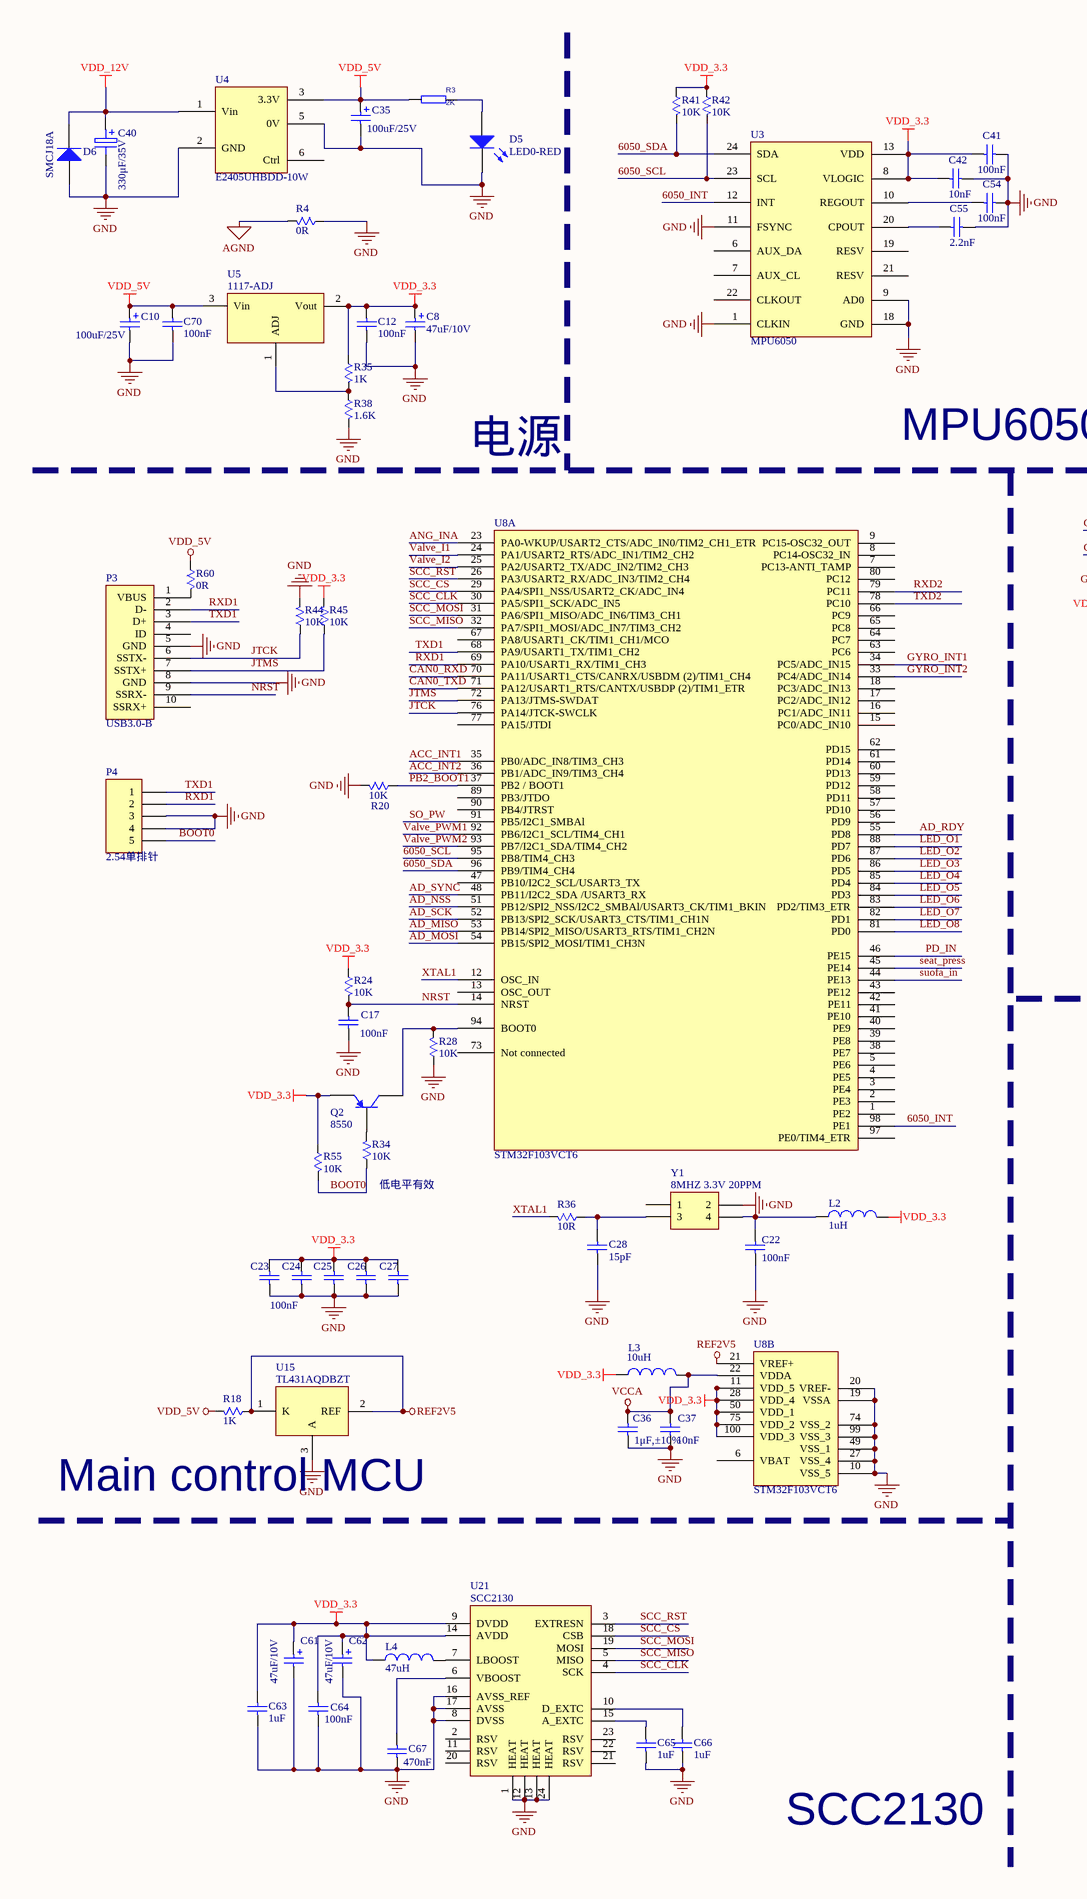
[diagram p0: MISC82155-6.SchDoc, left]
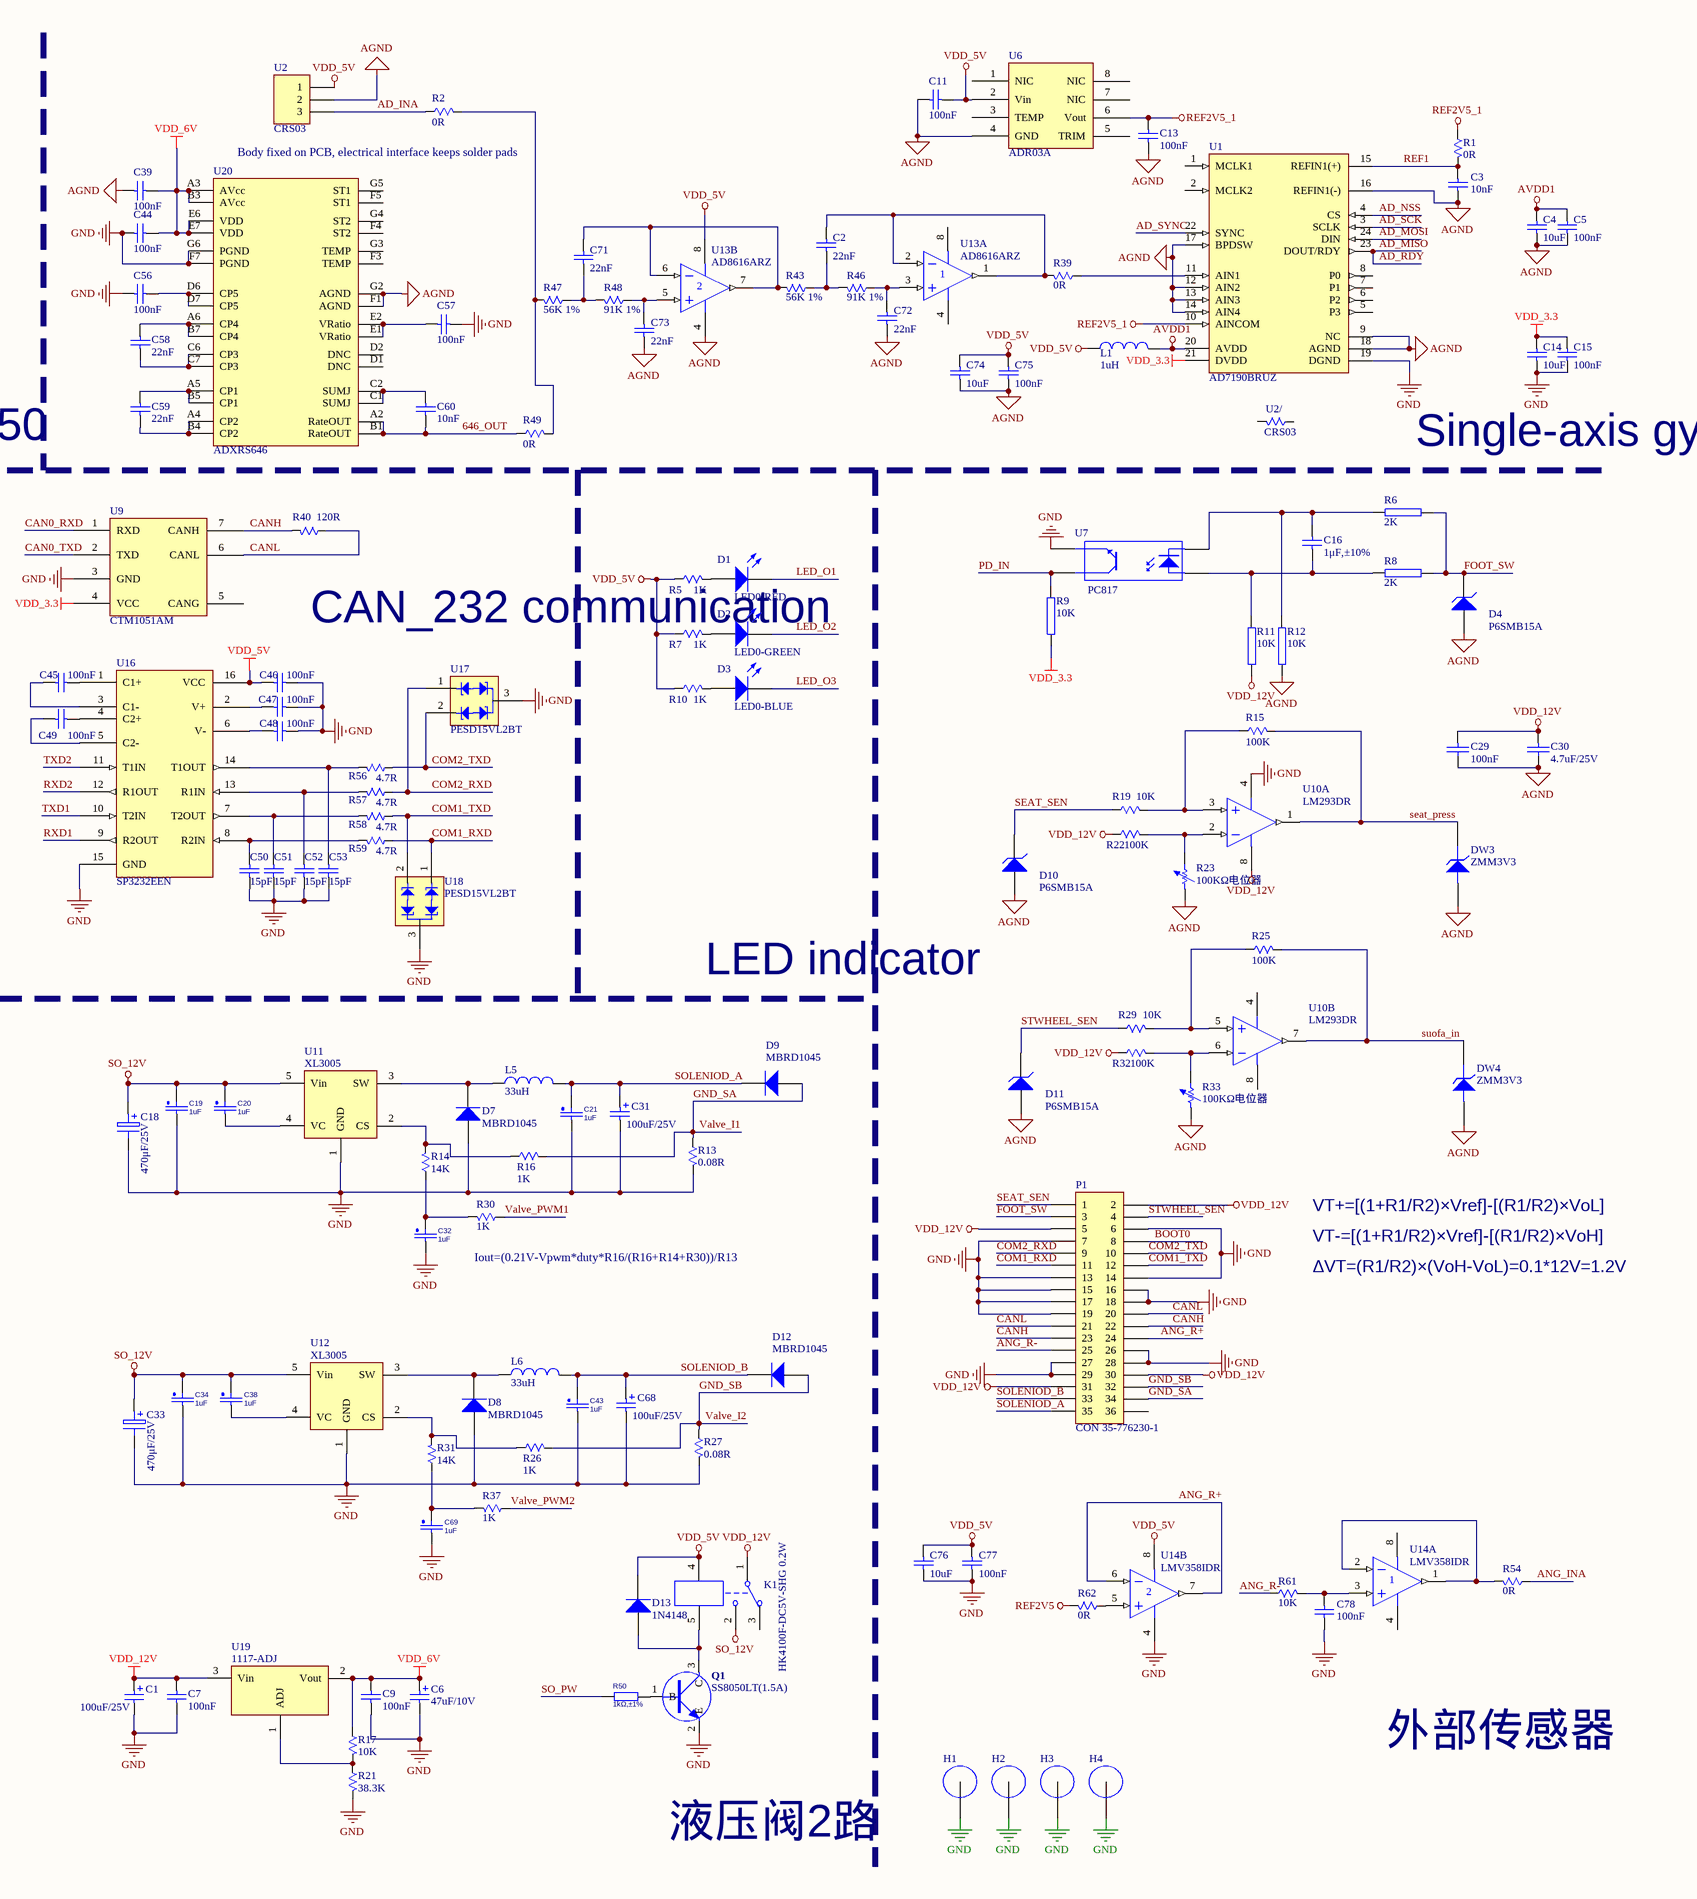
[diagram p1: MISC82155-6.SchDoc, right]
# Altium schematic sheet MISC82155-6.SchDoc
size A2

## Parts
C1  100uF/25V  [RB6.3*7]
C2  22nF  [C0805]
C3  10nF  [C0805]
C4  10uF  [C0805]
C5  100nF  [C0805]
C6  47uF/10V  [CT3528-B]
C7  100nF  [C0805]
C8  47uF/10V  [CT3528-B]
C9  100nF  [C0805]
C10  100uF/25V  [RB6.3*7]
C11  100nF  [C0805]
C12  100nF  [C0805]
C13  100nF  [C0805]
C14  10uF  [C0805]
C15  100nF  [C0805]
C16  1μF,±10%  [C0805]
C17  100nF  [C0805]
C18  470μF/25V  [CAPPR5.0-10X16-0.8]
C19  1uF  [C0805]
C20  1uF  [C0805]
C21  1uF  [C0805]
C22  100nF  [C0805]
C23  100nF  [C0805]
C24  100nF  [C0805]  (value not drawn)
C25  100nF  [C0805]  (value not drawn)
C26  100nF  [C0805]  (value not drawn)
C27  100nF  [C0805]  (value not drawn)
C28  15pF  [C0805]
C29  100nF  [C0805]
C30  4.7uF/25V  [1206C]
C31  100uF/25V  [RB6.3*7]
C32  1uF  [C0805]
C33  470μF/25V  [CAPPR5.0-10X16-0.8]
C34  1uF  [C0805]
C35  100uF/25V  [RB6.3*7]
C36  1μF,±10%  [C0805]
C37  10nF  [C0805]
C38  1uF  [C0805]
C39  100nF  [C0805]
C40  330μF/35V  [CAPPR5.0-10X16-0.8]
C41  100nF  [C0805]
C42  10nF  [C0805]
C43  1uF  [C0805]
C44  100nF  [C0805]
C45  100nF  [C0805]
C46  100nF  [C0805]
C47  100nF  [C0805]
C48  100nF  [C0805]
C49  100nF  [C0805]
C50  15pF  [C0805]
C51  15pF  [C0805]
C52  15pF  [C0805]
C53  15pF  [C0805]
C54  100nF  [C0805]
C55  2.2nF  [C0805]
C56  100nF  [C0805]
C57  100nF  [C0805]
C58  22nF  [C0805]
C59  22nF  [C0805]
C60  10nF  [C0805]
C61  47uF/10V  [CT3528-B]
C62  47uF/10V  [CT3528-B]
C63  1uF  [C0805]
C64  100nF  [C0805]
C65  1uF  [C0805]
C66  1uF  [C0805]
C67  470nF  [C0805]
C68  100uF/25V  [RB6.3*7]
C69  1uF  [C0805]
C70  100nF  [C0805]
C71  22nF  [C0805]
C72  22nF  [C0805]
C73  22nF  [C0805]
C74  10uF  [C0805]
C75  100nF  [C0805]
C76  10uF  [C0805]
C77  100nF  [C0805]
C78  100nF  [C0805]
D1  LED0-RED  [LED0805]
D2  LED0-GREEN  [LED0805]
D3  LED0-BLUE  [LED0805]
D4  P6SMB15A  [DO-214]
D5  LED0-RED  [LED0805]
D6  SMCJ18A  [SMC]
D7  MBRD1045  [TO-252]
D8  MBRD1045  [TO-252]
D9  MBRD1045  [TO-252]
D10  P6SMB15A  [DO-214]
D11  P6SMB15A  [DO-214]
D12  MBRD1045  [TO-252]
D13  1N4148  [SMD-D4148]
DW3  ZMM3V3  [SMD-D4148]
DW4  ZMM3V3  [SMD-D4148]
H1  Hole  [HOLE-3.2]  (value not drawn)
H2  Hole  [HOLE-3.2]  (value not drawn)
H3  Hole  [HOLE-3.2]  (value not drawn)
H4  Hole  [HOLE-3.2]  (value not drawn)
K1  HK4100F-DC5V-SHG 0.2W  [HK4100F]
L1  1uH  [R0805]
L2  1uH  [R0805]
L3  10uH  [R0805]
L4  47uH  [R1210]
L5  33uH  [SLF12555]
L6  33uH  [SLF12555]
P1  CON 35-776230-1  [VGA35]
P3  USB3.0-B  [Micro USB3.0-B]
P4  2.54单排针  [HDR1X5]
Q1  SS8050LT(1.5A)  [SOT-23]
Q2  8550  [SOT-23]
R1  0R  [R0805]
R2  0R  [R0805]
R3  2K  [R0805]
R4  0R  [R0805]
R5  1K  [R0805]
R6  2K  [R0805]
R7  1K  [R0805]
R8  2K  [R0805]
R9  10K  [R0805]
R10  1K  [R0805]
R11  10K  [R0805]
R12  10K  [R0805]
R13  0.08R  [R2512]
R14  14K  [R0805]
R15  100K  [R0805]
R16  1K  [R0805]
R17  10K  [R0805]
R18  1K  [R0805]
R19  10K  [R0805]
R20  10K  [R0805]
R21  38.3K  [R0805]
R22  100K  [R0805]
R23  100KΩ电位器  [CHANGER3]
R24  10K  [R0805]
R25  100K  [R0805]
R26  1K  [R0805]
R27  0.08R  [R2512]
R28  10K  [R0805]
R29  10K  [R0805]
R30  1K  [R0805]
R31  14K  [R0805]
R32  100K  [R0805]
R33  100KΩ电位器  [CHANGER3]
R34  10K  [R0805]
R35  1K  [R0805]
R36  10R  [R0805]
R37  1K  [R0805]
R38  1.6K  [R0805]
R39  0R  [R0805]
R40  120R  [R0805]
R41  10K  [R0805]
R42  10K  [R0805]
R43  56K 1%  [R0805]
R44  10K  [R0805]
R45  10K  [R0805]
R46  91K 1%  [R0805]
R47  56K 1%  [R0805]
R48  91K 1%  [R0805]
R49  0R  [R0805]
R50  1kΩ,±1%  [0805R]
R54  0R  [R0805]
R55  10K  [R0805]
R56  4.7R  [R0805]
R57  4.7R  [R0805]
R58  4.7R  [R0805]
R59  4.7R  [R0805]
R60  0R  [R0805]
R61  10K  [R0805]
R62  0R  [R0805]
U1  AD7190BRUZ  [IC-24P-TSSOP-6_4MM-G]
U2  CRS03  [HDR1X3]
U2/  CRS03  [CDS43-01]
U3  MPU6050  [QFN24]
U4  E2405UHBDD-10W  [E2403UHBDD]
U5  1117-ADJ  [SOT-223]
U6  ADR03A  [SOP-8]
U7  PC817  [SMD-4]
U8  STM32F103VCT6  [QFP-100]  (parts A,B of 2)
U9  CTM1051AM  [CTM1051AM]
U10  LM293DR  [SOP-8]  (parts A,B of 2)
U11  XL3005  [TO-263-5]
U12  XL3005  [TO-263-5]
U13  AD8616ARZ  [SOP-8]  (parts A,B of 2)
U14  LMV358IDR  [SOP-8]  (parts A,B of 2)
U15  TL431AQDBZT  [LC-SOT-23(SOT-23-3)]
U16  SP3232EEN  [SOP16-6.6]
U17  PESD15VL2BT  [SOT-23]
U18  PESD15VL2BT  [SOT-23]
U19  1117-ADJ  [SOT-223]
U20  ADXRS646
U21  SCC2130  [SCC2130D]
Y1  8MHZ 3.3V 20PPM  [XTAL7050]

## Nets
AGND: C3.2 C4.2 C5.2 C11.1 C13.2 C29.2 C30.2 C39.1 C72.2 C73.2 C74.2 C75.2 D4.1(A) D10.1(A) D11.1(A) DW3.1(A) DW4.1(A) R4.1 R12.2 R23.1 R33.1 U1.9(NC) U1.12(AIN2) U1.13(AIN3) U1.14(AIN4) U1.16(REFIN1(-)) U1.17(BPDSW) U1.18(AGND) U2.2 U6.4(GND) U13.4(V-) U20.F1(AGND) U20.G2(AGND)
AVDD1: C4.1 C5.1 L1.2 U1.20(AVDD)
GND: C1.2 C6.2 C7.1 C8.2 C9.1 C10.2 C12.1 C14.2 C15.2 C17.1 C18.2 C19.2 C21.2 C22.2 C23.2 C24.2 C25.2 C26.2 C27.2 C28.1 C31.2 C32.2 C33.2 C34.2 C35.2 C36.1 C37.1 C40.2 C41.1 C42.1 C43.2 C44.1 C46.2 C47.2 C48.2 C50.2 C51.2 C52.2 C53.2 C54.1 C55.1 C56.1 C57.2 C61.2 C62.2 C63.2 C64.2 C65.2 C66.2 C67.2 C68.2 C69.2 C70.1 C76.2 C77.2 C78.2 D5.2(K) D6.1(A) D7.1(A) D8.1(A) H1.8(CANH) H2.8(CANH) H3.8(CANH) H4.8(CANH) P1.6 P1.7 P1.13 P1.14 P1.15 P1.16 P1.17 P1.18 P1.19 P1.26 P1.27 P1.28 P1.29 P3.5(GND) P3.8(GND) P4.3 P4.4 Q1.2(E) R4.2 R13.1 R20.1 R21.1 R27.1 R28.1 R38.1 R44.1 U1.19(DGND) U3.1(CLKIN) U3.9(AD0) U3.11(FSYNC) U3.18(GND) U4.2(GND) U4.5(0V) U7.3(E) U8.10(VSS_5) U8.19(VSSA) U8.20(VREF-) U8.27(VSS_4) U8.49(VSS_1) U8.74(VSS_2) U8.99(VSS_3) U9.3(GND) U10.4(GND) U11.1(GND) U12.1(GND) U14.4(V-) U15.3(A) U16.15(GND) U17.3 U18.3 U20.F7(PGND) U20.G6(PGND) U21.1(HEAT) U21.8(DVSS) U21.12(HEAT) U21.13(HEAT) U21.16(AVSS_REF) U21.17(AVSS) U21.24(HEAT) Y1.2
REF2V5: R18.2 R62.1 U8.21(VREF+) U15.1(K) U15.2(REF)
REF2V5_1: C13.1 R1.2 U1.10(AINCOM) U6.6(Vout)
SO_12V: C18.1 C19.1 C20.1 C33.1 C34.1 C38.1 K1.2 U11.5(Vin) U12.5(Vin)
VCCA: C36.2 C37.2 L3.2 U8.22(VDDA)
VDD_3.3: C8.1 C12.2 C14.1 C15.1 C23.1 C24.1 C25.1 C26.1 C27.1 C41.2 C42.2 C61.1 C62.1 C63.1 C64.1 L2.2 L3.1 L4.1 Q2.2(E) R9.1 R24.2 R35.2 R41.2 R42.2 R45.1 R55.2 U1.21(DVDD) U3.8(VLOGIC) U3.13(VDD) U5.2(Vout) U8.11(VDD_5) U8.28(VDD_4) U8.50(VDD_1) U8.75(VDD_2) U8.100(VDD_3) U9.4(VCC) U21.9(DVDD) U21.14(AVDD)
VDD_5V: C10.1 C11.2 C35.1 C46.1 C70.2 C74.1 C75.1 C76.1 C77.1 D13.2(K) K1.4 L1.1 R3.2 R5.2 R7.2 R10.2 R18.1 R60.1 U2.1 U4.3(3.3V) U5.3(Vin) U6.2(Vin) U13.8(V+) U14.8(V+) U16.16(VCC)
VDD_6V: C6.1 C9.2 C39.2 C44.2 R17.2 U19.2(Vout) U20.A3(AVcc) U20.B3(AVcc) U20.E6(VDD) U20.E7(VDD)
VDD_12V: C1.1 C7.2 C29.1 C30.1 C40.1 D6.2(K) K1.1 P1.2 P1.5 P1.30 P1.31 R11.2 R22.2 R32.2 U4.1(Vin) U10.8(V+) U19.3(Vin)
646_OUT: C60.1 R49.2 U20.A2(RateOUT) U20.B1(RateOUT)
6050_INT: U3.12(INT) U8.98(PE1)
6050_SCL: R42.1 U3.23(SCL) U8.95(PB8/TIM4_CH3)
6050_SDA: R41.1 U3.24(SDA) U8.96(PB9/TIM4_CH4)
ACC_INT1: U8.35(PB0/ADC_IN8/TIM3_CH3)
ACC_INT2: U8.36(PB1/ADC_IN9/TIM3_CH4)
AD_INA: R2.2 U2.3
AD_MISO: U1.23(DOUT/RDY) U8.53(PB14/SPI2_MISO/USART3_RTS/TIM1_CH2N) U8.55(PD8)  [also labelled AD_RDY]
AD_MOSI: U1.24(DIN) U8.54(PB15/SPI2_MOSI/TIM1_CH3N)
AD_NSS: U1.4(CS) U8.51(PB12/SPI2_NSS/I2C2_SMBAl/USART3_CK/TIM1_BKIN)
AD_SCK: U1.3(SCLK) U8.52(PB13/SPI2_SCK/USART3_CTS/TIM1_CH1N)
AD_SYNC: U1.22(SYNC) U8.48(PB11/I2C2_SDA_/USART3_RX)
ANG_INA: R54.2 U8.23(PA0-WKUP/USART2_CTS/ADC_IN0/TIM2_CH1_ETR)
ANG_R+: P1.24 U14.6(IN-) U14.7(OUT)
ANG_R-: P1.25 R61.2
BOOT0: P1.8 P4.5 R34.2 R55.1
CAN0_RXD: U8.70(PA11/USART1_CTS/CANRX/USBDM_(2)/TIM1_CH4) U9.1(RXD)
CAN0_TXD: U8.71(PA12/USART1_RTS/CANTX/USBDP_(2)/TIM1_ETR) U9.2(TXD)
CANH: P1.22 P1.23 R40.1 U9.7(CANH)
CANL: P1.20 P1.21 R40.2 U9.6(CANL)
COM1_RXD: P1.11 R59.2 U18.1
COM1_TXD: P1.12 R58.2 U18.2
COM2_RXD: P1.9 R57.2 U17.1
COM2_TXD: P1.10 R56.2 U17.2
FOOT_SW: D4.2(K) P1.3 R6.1 R8.1
GND_SA: D9.1(A) P1.34 R13.2 R16.1 U8.24(PA1/USART2_RTS/ADC_IN1/TIM2_CH2)  [also labelled Valve_I1]
GND_SB: D12.1(A) P1.32 R26.1 R27.2 U8.25(PA2/USART2_TX/ADC_IN2/TIM2_CH3)  [also labelled Valve_I2]
GYRO_INT1: U8.34(PC5/ADC_IN15)
GYRO_INT2: U8.33(PC4/ADC_IN14)
JTCK: P3.6(SSTX-) R44.2 U8.76(PA14/JTCK-SWCLK)
JTMS: P3.7(SSTX+) R45.2 U8.72(PA13/JTMS-SWDAT)
LED_O1: D1.2(K) U8.88(PD7)
LED_O2: D2.2(K) U8.87(PD6)
LED_O3: D3.2(K) U8.86(PD5)
LED_O4: U8.85(PD4)
LED_O5: U8.84(PD3)
LED_O6: U8.83(PD2/TIM3_ETR)
LED_O7: U8.82(PD1)
LED_O8: U8.81(PD0)
NRST: C17.2 P3.9(SSRX-) R24.1 U8.14(NRST)
PB2_BOOT1: R20.2 U8.37(PB2_/_BOOT1)
PD_IN: R9.2 U7.4(C) U8.46(PE15)
REF1: C3.1 R1.1 U1.15(REFIN1(+))
RXD1: P3.2(D-) P4.2 U8.69(PA10/USART1_RX/TIM1_CH3) U16.9(R2OUT)
RXD2: U8.79(PC11) U16.12(R1OUT)
SCC_CLK: U8.30(PA5/SPI1_SCK/ADC_IN5) U21.4(SCK)
SCC_CS: U8.29(PA4/SPI1_NSS/USART2_CK/ADC_IN4) U21.18(CSB)
SCC_MISO: U8.32(PA7/SPI1_MOSI/ADC_IN7/TIM3_CH2) U21.5(MISO)
SCC_MOSI: U8.31(PA6/SPI1_MISO/ADC_IN6/TIM3_CH1) U21.19(MOSI)
SCC_RST: U8.26(PA3/USART2_RX/ADC_IN3/TIM2_CH4) U21.3(EXTRESN)
seat_press: DW3.2(K) R15.1 U8.45(PE14) U10.1(OUT)
SEAT_SEN: D10.2(K) P1.1 R19.2
SO_PW: R50.1 U8.91(PB5/I2C1_SMBAl)
SOLENIOD_A: C21.1 C31.1 D9.2(K) L5.2 P1.35
SOLENIOD_B: C43.1 C68.1 D12.2(K) L6.2 P1.33
STWHEEL_SEN: D11.2(K) P1.4 R29.2
suofa_in: DW4.2(K) R25.1 U8.44(PE13) U10.7(OUT)
TXD1: P3.3(D+) P4.1 U8.68(PA9/USART1_TX/TIM1_CH2) U16.10(T2IN)
TXD2: U8.78(PC10) U16.11(T1IN)
Valve_PWM1: R30.1 U8.92(PB6/I2C1_SCL/TIM4_CH1)
Valve_PWM2: R37.1 U8.93(PB7/I2C1_SDA/TIM4_CH2)
XTAL1: R36.1 U8.12(OSC_IN)
NetC2_1: C2.1 R39.1 U13.1(OUT) U13.2(IN-)
NetC2_2: C2.2 R43.2 R46.1
NetC16_1: C16.1 R8.2 R11.1 U7.1(A)
NetC16_2: C16.2 R6.2 R12.1 U7.2(K)
NetC20_2: C20.2 U11.4(VC)
NetC22_1: C22.1 L2.1 Y1.4
NetC28_2: C28.2 R36.2 Y1.3
NetC32_1: C32.1 R14.2 R30.2
NetC38_2: C38.2 U12.4(VC)
NetC45_1: C45.1 U16.3(C1-)
NetC45_2: C45.2 U16.1(C1+)
NetC47_1: C47.1 U16.2(V+)
NetC48_1: C48.1 U16.6(V-)
NetC49_1: C49.1 U16.5(C2-)
NetC49_2: C49.2 U16.4(C2+)
NetC50_1: C50.1 R59.1 U16.8(R2IN)
NetC51_1: C51.1 R58.1 U16.7(T2OUT)
NetC52_1: C52.1 R57.1 U16.13(R1IN)
NetC53_1: C53.1 R56.1 U16.14(T1OUT)
NetC54_2: C54.2 U3.10(REGOUT)
NetC55_2: C55.2 U3.20(CPOUT)
NetC56_2: C56.2 U20.D6(CP5) U20.D7(CP5)
NetC57_1: C57.1 U20.E1(VRatio) U20.E2(VRatio)
NetC58_1: C58.1 U20.A6(CP4) U20.B7(CP4)
NetC58_2: C58.2 U20.C6(CP3) U20.C7(CP3)
NetC59_1: C59.1 U20.A5(CP1) U20.B5(CP1)
NetC59_2: C59.2 U20.A4(CP2) U20.B4(CP2)
NetC60_2: C60.2 U20.C1(SUMJ) U20.C2(SUMJ)
NetC65_1: C65.1 U21.15(A_EXTC)
NetC66_1: C66.1 U21.10(D_EXTC)
NetC67_1: C67.1 U21.6(VBOOST)
NetC69_1: C69.1 R31.2 R37.2
NetC71_1: C71.1 R43.1 U13.6(IN-) U13.7(OUT)
NetC71_2: C71.2 R47.2 R48.1
NetC72_1: C72.1 R46.2 U13.3(IN+)
NetC73_1: C73.1 R48.2 U13.5(IN+)
NetC78_1: C78.1 R61.1 U14.3(IN+)
NetD1_1: D1.1(A) R5.1
NetD2_1: D2.1(A) R7.1
NetD3_1: D3.1(A) R10.1
NetD5_1: D5.1(A) R3.1
NetD7_2: D7.2(K) L5.1 U11.3(SW)
NetD8_2: D8.2(K) L6.1 U12.3(SW)
NetD13_1: D13.1(A) K1.5 Q1.3(C)
NetL4_2: L4.2 U21.7(LBOOST)
NetP3_1: P3.1(VBUS) R60.2
NetQ1_1: Q1.1(B) R50.2
NetQ2_1: Q2.1(B) R34.1
NetQ2_3: Q2.3(C) R28.2 U8.94(BOOT0)
NetR2_1: R2.1 R47.1 R49.1
NetR14_1: R14.1 R16.2 U11.2(CS)
NetR15_2: R15.2 R19.1 U10.3(IN+)
NetR17_1: R17.1 R21.2 U19.1(ADJ)
NetR22_1: R22.1 R23.2 U10.2(IN-)
NetR25_2: R25.2 R29.1 U10.5(IN+)
NetR26_2: R26.2 R31.1 U12.2(CS)
NetR32_1: R32.1 R33.2 U10.6(IN-)
NetR35_1: R35.1 R38.2 U5.1(ADJ)
NetR39_2: R39.2 U1.11(AIN1)
NetR54_1: R54.1 U14.1(OUT) U14.2(IN-)
NetR62_2: R62.2 U14.5(IN+)

Not connected (* = marked no-connect by the designer): K1 3(2); P1 36; P3 4(ID) 10(SSRX+); U1 1(MCLK1) 2(MCLK2) 5(P3) 6(P2) 7(P1) 8(P0); U2/ 1 2; U3 6(AUX_DA) 7(AUX_CL) 19(RESV) 21(RESV) 22(CLKOUT); U4 6(Ctrl); U6 1(NIC) 3(TEMP) 5(TRIM) 7(NIC) 8(NIC); U8 1(PE2) 2(PE3) 3(PE4) 4(PE5) 5(PE6) 6(VBAT) 7(PC13-ANTI_TAMP) 8(PC14-OSC32_IN) 9(PC15-OSC32_OUT) 13(OSC_OUT) 15(PC0/ADC_IN10) 16(PC1/ADC_IN11) 17(PC2/ADC_IN12) 18(PC3/ADC_IN13) 38(PE7) 39(PE8) 40(PE9) 41(PE10) 42(PE11) 43(PE12) 47(PB10/I2C2_SCL/USART3_TX) 56(PD9) 57(PD10) 58(PD11) 59(PD12) 60(PD13) 61(PD14) 62(PD15) 63(PC6) 64(PC7) 65(PC8) 66(PC9) 67(PA8/USART1_CK/TIM1_CH1/MCO) 73(Not_connected) 77(PA15/JTDI) 80(PC12) 89(PB3/JTDO) 90(PB4/JTRST) 97(PE0/TIM4_ETR); U9 5(CANG); U20 D1(DNC) D2(DNC) F3(TEMP) F4(ST2) F5(ST1) G3(TEMP) G4(ST2) G5(ST1); U21 2(RSV) 11(RSV) 20(RSV) 21(RSV) 22(RSV) 23(RSV); Y1 1

## Notes on the sheet
- Body fixed on PCB, electrical interface keeps solder pads
- 电源
- MPU6050
- Single-axis gyro
- CAN_232 communication
- LED indicator
- (near R34) 低电平有效
- VT+=[(1+R1/R2)×Vref]-[(R1/R2)×VoL]
- VT-=[(1+R1/R2)×Vref]-[(R1/R2)×VoH]
- Iout=(0.21V-Vpwm*duty*R16/(R16+R14+R30))/R13
- ΔVT=(R1/R2)×(VoH-VoL)=0.1*12V=1.2V
- (near U15) Main control MCU
- 外部传感器
- SCC2130
- 液压阀2路

## Library data of the parts
C1 C6 C8 C10 C31 C35 C61 C62 C68 = Cap Pol2: Polarized Capacitor (Axial); Published: 8-Jun-2000; LatestRevisionDate: 17-Jul-2002; LatestRevisionNote: Re-released for DXP Platform.; PackageReference: POLAR0.8; PackageDescription: Polarized Capacitor; 2 Leads; Publisher: Altium Limited
  C1 C10 C31 C35 C68: Value: 100uF/25V
  C6 C8 C61 C62: Value: 47uF/10V
C2 C22 C71-C73 C75 C77 C78 = Cap: Capacitor; Value: 10nF; Published: 8-Jun-2000; Revision: July-2002: Re-released for DXP Platform.; Publisher: Altium Limited
C3-C5 C7 C9 C11-C17 C23-C28 C36 C37 C39 C41 C42 C44-C60 C63-C67 C70 C74 C76 = Cap: Capacitor; Published: 8-Jun-2000; Revision: July-2002: Re-released for DXP Platform.; Publisher: Altium Limited
  C3 C37 C42 C60: Value: 10nF
  C4 C14 C74 C76: Value: 10uF
  C5 C7 C9 C11-C13 C15 C17 C23-C27 C39 C41 C44-C49 C54 C56 C57 C64 C70: Value: 100nF
  C16 C36: Value: 1μF,±10%
  C28 C50-C53: Value: 15pF
  C55: Value: 2.2nF
  C58 C59: Value: 22nF
  C63 C65 C66: Value: 1uF
  C67: Value: 470nF
C18 C33 C40 = 1.02.11.0018: 220μF,16V,Ф6.3×7mm,,珠海华冠,RoHS; 名称: 电解电容; 贴片和直插: THT; 器件优选方案: 状态正常; PCB备注: Fcqh-Slq-Twrj-141216; 物料代码: 1.02.11.0018; 厂商: 珠海华冠; RoHS: RoHS; 型号: 220μF,16V,Ф6.3×7mm; ComponentLink1Description: ErpDataInfo
  C18 C33: Value: 470μF/25V
  C40: Value: 330μF/35V
C19-C21 C32 C34 C38 C43 C69 = CAP NP_Dup5: Value: 1uF
C29 C30 = CAP: Capacitor
  C29: Value: 100nF
  C30: Value: 4.7uF/25V
D1-D3 D5 = LED0: Typical INFRARED GaAs LED; Published: 8-Jun-2000; LatestRevisionDate: 08-Jul-2005; LatestRevisionNote: Mech Layer 1 removed.; PackageReference: LED-0; PackageDescription: LED; 2 Leads; Publisher: Altium Limited
D4 D10 D11 = D Zener: Zener Diode; Published: 8-Jun-2000; LatestRevisionDate: 17-Jul-2002; LatestRevisionNote: Re-released for DXP Platform.; PackageReference: DIODE-0.7; Publisher: Altium Limited
D6-D9 D12 = Diode 1N4007: 1 Amp General Purpose Rectifier; Published: 8-Jun-2000; LatestRevisionDate: 17-Jul-2002; LatestRevisionNote: Re-released for DXP Platform.; DatasheetVersion: 1998; PackageVersion: Aug-1999; PackageReference: DO-41; PackageDescription: Diode, Axial; Body 5.2 x 2.7 mm (LxDia. max), Lead Dia. 0.86 mm (max); Code_JEDEC: DO-204-AL; ComponentLink1Description: Manufacturer Link; ComponentLink2Description: Datasheet; ComponentLink2URL: http://www.fairchildsemi.com/ds/1N%2F1N4001.pdf; Publisher: Altium Limited
D13 = Diode: Default Diode; Published: 8-Jun-2000; LatestRevisionDate: 17-Jul-2002; LatestRevisionNote: Re-released for DXP Platform.; PackageVersion: Sep-1996; PackageReference: SMC; PackageDescription: DO-214-AB/SMC; 2 C-Bend Leads; Body 7.9 x 5.9 mm, inc. leads (LxW); Code_JEDEC: DO-214-AB; Publisher: Altium Limited
DW3 DW4 = ZENER3: Zener Diode
K1 = Relay-SPDT: Single-Pole Dual-Throw Relay; Published: 24-Mar-1999; LatestRevisionDate: 17-Jul-2002; LatestRevisionNote: Re-released for DXP Platform.; PackageReference: MODULE5B; Publisher: Altium Limited
L1-L6 = Inductor: Code_IEC: 1005; Published: 8-Jun-2000; PackageReference: 0402-A; Code_JEITA: 0402; Publisher: Altium Limited
  L1 L2: LatestRevisionDate: 17-Jul-2002; LatestRevisionNote: Re-released for DXP Platform.; Value: 1uH
  L3: LatestRevisionDate: 17-Jul-2002; LatestRevisionNote: Re-released for DXP Platform.; Value: 10uH
  L4: LatestRevisionDate: 29-May-2009; LatestRevisionNote: IPC-7351 Footprint Added.; PackageDescription: Chip Inductor; Value: 47uH
  L5 L6: LatestRevisionDate: 29-May-2009; LatestRevisionNote: IPC-7351 Footprint Added.; PackageDescription: Chip Inductor; Value: 33uH
P1 = Header 18X2: Header, 18-Pin, Dual row; LatestRevisionDate: 17-Jul-2002; LatestRevisionNote: Re-released for DXP Platform.; Publisher: Altium Limited
P4 = Header 5: Header, 5-Pin; LatestRevisionDate: 17-Jul-2002; LatestRevisionNote: Re-released for DXP Platform.; Publisher: Altium Limited
Q1 = 1.04.09.0001: SS8050LT(1.5A),SOT-23,Jiangsu Changdian,RoHS; 名称: 三极管; 设备封装名称: SOT-23_SS8050LT; 厂商: 江苏长电; 贴片和直插: SMT; 物料代码: 1.04.09.0001; Value: SS8050LT(1.5A); 封装: SOT-23; RoHS: RoHS; 型号: SS8050LT(1.5A); ComponentLink1Description: ErpDataInfo
Q2 = PNP: PNP Bipolar Transistor; Published: 8-Jun-2000; LatestRevisionDate: 29-May-2009; LatestRevisionNote: IPC-7351 Footprint Added.; PackageVersion: Aug-1999; PackageReference: SOT-23B; PackageDescription: 3-Pin SOT-23 Package 0.95 mm Pitch, 2.4 mm Lead Span; Publisher: Altium Limited
R1 R2 R4 R5 R7 R10 R13-R22 R24-R32 R34-R49 R54-R62 = Res: Resistor; Published: 8-Jun-2000; LatestRevisionDate: 04-Mar-2005; LatestRevisionNote: PCB Footprint replaced.; PackageReference: J1-0603; Publisher: Altium Limited
  R1 R2 R4 R39 R49 R54 R60 R62: Value: 0R
  R5 R7 R10 R16 R18 R26 R30 R35 R37: Value: 1K
  R13 R27: Value: 0.08R
  R14 R31: Value: 14K
  R15 R22 R25 R32: Value: 100K
  R17 R19 R20 R24 R28 R29 R34 R41 R42 R44 R45 R55 R61: Value: 10K
  R21: Value: 38.3K
  R36: Value: 10R
  R38: Value: 1.6K
  R40: Value: 120R
  R43 R47: Value: 56K 1%
  R46 R48: Value: 91K 1%
  R56-R59: Value: 4.7R
R3 R50 = RES
  R50: Value: 1kΩ,±1%
R6 R8 R11 R12 = 1.01.17.0004: 名称: 电阻; 封装: 0402; 设备封装名称: R0402_0R; 型号: 1k ohm,±1%; 贴片和直插: SMT; 厂商: RALEC; 物料代码: 1.01.17.0004; RoHS: RoHS; ComponentLink1Description: ErpDataInfo
  R6 R8: Value: 2K
  R11 R12: Value: 10K
R9 = 1.01.17.0004: 名称: 电阻; 封装: 0402; 设备封装名称: R0402_0R; 型号: 0Ω,±1%; 贴片和直插: SMT; 厂商: RALEC; 物料代码: 1.01.17.0004; Value: 10K; RoHS: RoHS; ComponentLink1Description: ErpDataInfo
R23 R33 = Res Adj1: Variable Resistor; Set Position: 0.5; Published: 8-Jun-2000; LatestRevisionDate: 17-Jul-2002; LatestRevisionNote: Re-released for DXP Platform.; PackageReference: AXIAL-0.7; PackageDescription: Axial Device, Thru-Hole; 2 Leads; 0.7 in Pin Spacing; Value: 100KΩ电位器; Publisher: Altium Limited
U1 = AD7190
U2 = Header 3: Header, 3-Pin; LatestRevisionDate: 17-Jul-2002; LatestRevisionNote: Re-released for DXP Platform.; Publisher: Altium Limited
U2/ = Res: Resistor; Value: 10R; Published: 8-Jun-2000; LatestRevisionDate: 04-Mar-2005; LatestRevisionNote: PCB Footprint replaced.; PackageReference: J1-0603; Publisher: Altium Limited
U3 = ITG3050: 3-axi gyros
U4 = E2403UHBDD-10W
U5 U19 = VOLTREG1
U6 = ADR03ARZ
U7 = TLP281-1: Optoisolator
U8 = STM32F103VBH6
U10 = LM293D: Dual Comparator; Published: 17-Jul-2002; LatestRevisionDate: 13-Apr-2006; LatestRevisionNote: IPC-7351 Footprint Added.; DatasheetVersion: 1988; PackageReference: 751-02; PackageDescription: 8-Pin Small Outline Integrated Circuit 1.27 mm Pitch; Code_JEDEC: MS-012-AA; Code_IPC: SOIC127P600-8; ComponentLink1Description: Manufacturer Link; ComponentLink1URL: http://www.onsemi.com/site/products/taxonomy/0,4438,133,00.html; Publisher: Altium Limited
U13 U14 = LM358D: Dual Low-Power Operational Amplifier; Published: 17-Jul-2002; LatestRevisionDate: 13-Apr-2006; LatestRevisionNote: IPC-7351 Footprint Added.; DatasheetVersion: 1988; PackageReference: 751-02; PackageDescription: 8-Pin Small Outline Integrated Circuit 1.27 mm Pitch; Code_JEDEC: MS-012-AA; Code_IPC: SOIC127P600-8; ComponentLink1Description: Manufacturer Link; ComponentLink1URL: http://www.onsemi.com/site/products/parametrics/0,4446,251,00.html; ComponentLink2Description: Datasheet; ComponentLink2URL: http://www.onsemi.com/pub/Collateral/LM358-D.PDF; Publisher: Altium Limited
U15 = TL431A
U16 = SP202ECT
U17 U18 = PESD12VL2BT
Y1 = Header 2X2: Header, 2-Pin, Dual row; LatestRevisionDate: 17-Jul-2002; LatestRevisionNote: Re-released for DXP Platform.; Publisher: Altium Limited